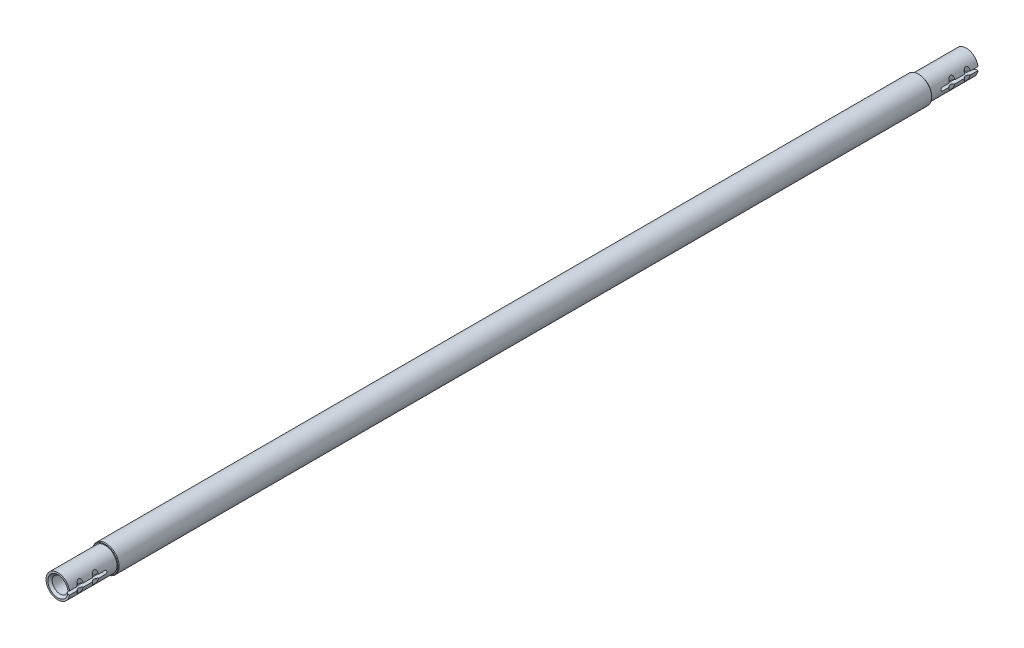
from build123d import *

# Parameters (mm, degrees)
SKETCH_2_R                    = 22.5
EXTRUDE_1_DEPTH               = 767.5
SKETCH_3_R                    = 22.5
SKETCH_3_R_2                  = 20
CUT_EXTRUDE_1_DEPTH           = 80
SKETCH_4_R                    = 16
CUT_EXTRUDE_2_DEPTH           = 30
CUT_EXTRUDE_3_REACH           = 1437.353
SKETCH_5_R                    = 12.5
HOLE_WIZARD_M30_1_D           = 26.5
HOLE_WIZARD_M30_1_DEPTH       = 70
HOLE_WIZARD_M30_1_CSINK_D     = 34
HOLE_WIZARD_M30_1_CSINK_ANGLE = 90
HOLE_WIZARD_M30_2_D           = 26.5
HOLE_WIZARD_M30_2_DEPTH       = 70
HOLE_WIZARD_M30_2_CSINK_D     = 34
HOLE_WIZARD_M30_2_CSINK_ANGLE = 90
SKETCH_10_R                   = 6
CUT_EXTRUDE_4_DEPTH           = 769.159325921
CUT_EXTRUDE_5_DEPTH           = 769.159326021
CHAMFER_1_SIZE                = 1


with BuildPart() as part:
    # 草图2 → 凸台-拉伸1 (new, symmetric)
    with BuildSketch(Plane.XY):
        Circle(SKETCH_2_R)
    extrude(amount=EXTRUDE_1_DEPTH, both=True)

    # 草图3 → 切除-拉伸1 (cut)
    with BuildSketch(Plane.XY.offset(767.5)):
        Circle(SKETCH_3_R)
        Circle(SKETCH_3_R_2, mode=Mode.SUBTRACT)
    cut_extrude_1 = extrude(amount=-CUT_EXTRUDE_1_DEPTH, mode=Mode.SUBTRACT)

    # 草图4 → 切除-拉伸2 (cut)
    with BuildSketch(Plane.XY.offset(667.5)):
        Circle(SKETCH_4_R)
    cut_extrude_2 = extrude(amount=CUT_EXTRUDE_2_DEPTH, mode=Mode.SUBTRACT)

    # 镜向1: 切除-拉伸1, 切除-拉伸2 across plane
    add(cut_extrude_1.mirror(Plane.XY), mode=Mode.SUBTRACT)
    add(cut_extrude_2.mirror(Plane.XY), mode=Mode.SUBTRACT)

    # 草图5 → 切除-拉伸3 (cut, up to next)
    with BuildSketch(Plane.XY.offset(667.5), mode=Mode.PRIVATE) as cut_extrude_3_sk1:
        Circle(SKETCH_5_R)
    cut_extrude_3_tool1 = extrude(cut_extrude_3_sk1.sketch, amount=-CUT_EXTRUDE_3_REACH, mode=Mode.PRIVATE) & part.part
    add(cut_extrude_3_tool1.solids().sort_by_distance((0, 0, 667.5))[0], mode=Mode.SUBTRACT)

    # M30 螺纹孔1
    with Locations(Plane.XY.offset(767.5)):
        with Locations((0, 0)):
            CounterSinkHole(HOLE_WIZARD_M30_1_D / 2, HOLE_WIZARD_M30_1_CSINK_D / 2, depth=HOLE_WIZARD_M30_1_DEPTH, counter_sink_angle=HOLE_WIZARD_M30_1_CSINK_ANGLE)

    # M30 螺纹孔2-左旋
    with Locations(Plane(origin=(0, 0, -767.5), x_dir=(-1, 0, 0), z_dir=(0, 0, -1))):
        with Locations((0, 0)):
            CounterSinkHole(HOLE_WIZARD_M30_2_D / 2, HOLE_WIZARD_M30_2_CSINK_D / 2, depth=HOLE_WIZARD_M30_2_DEPTH, counter_sink_angle=HOLE_WIZARD_M30_2_CSINK_ANGLE)

    # 草图10 → 切除-拉伸4 (cut, symmetric)
    with BuildSketch(Plane(origin=(0, 0, 0), x_dir=(1, 0, 0), z_dir=(0, 1, 0))):
        with Locations((23, -749.5)):
            Circle(SKETCH_10_R)
        with Locations((23, -723.5)):
            Circle(SKETCH_10_R)
    cut_extrude_4 = extrude(amount=CUT_EXTRUDE_4_DEPTH, both=True, mode=Mode.SUBTRACT)

    # 草图11 → 切除-拉伸5 (cut, through all)
    with BuildSketch(Plane(origin=(0, 0, 0), x_dir=(0, 0, -1), z_dir=(1, 0, 0))):
        with BuildLine():
            Line((-767.5, 3), (-707.5, 3))
            ThreePointArc((-707.5, 3), (-704.5, 0), (-707.5, -3))
            Line((-707.5, -3), (-767.5, -3))
            ThreePointArc((-767.5, -3), (-770.5, 0), (-767.5, 3))
        make_face()
    cut_extrude_5 = extrude(amount=CUT_EXTRUDE_5_DEPTH, mode=Mode.SUBTRACT)

    # 镜向2: 切除-拉伸4, 切除-拉伸5 across plane
    add(cut_extrude_4.mirror(Plane.XY), mode=Mode.SUBTRACT)
    add(cut_extrude_5.mirror(Plane.XY), mode=Mode.SUBTRACT)

    # 倒角1
    chamfer_1_edges = [part.edges().sort_by_distance(p)[0] for p in [
        (-22.5, 0, -687.5),
        (-22.5, 0, 687.5),
    ]]
    chamfer(chamfer_1_edges, length=CHAMFER_1_SIZE)


solid = part.part
